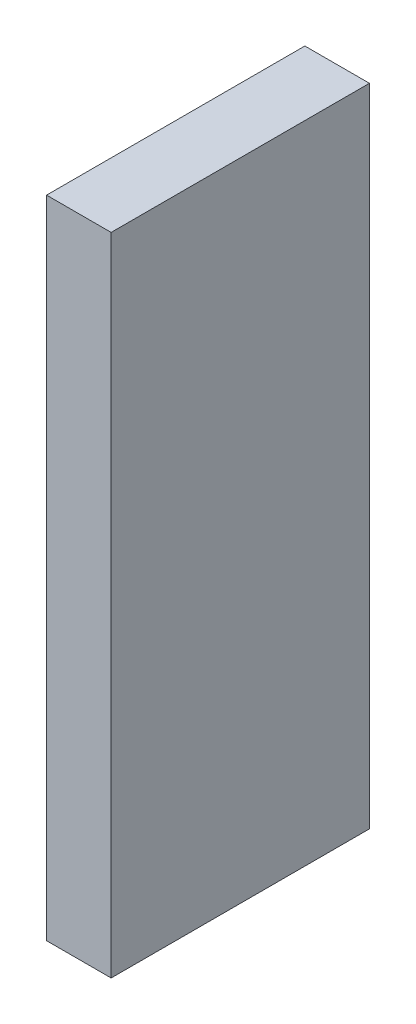
from build123d import *

# Parameters (mm, degrees)
SKETCH1_W           = 25
SKETCH1_H           = 250
BOSS_EXTRUDE1_DEPTH = 100


with BuildPart() as part:
    # Sketch1 → Boss-Extrude1 (new body)
    with BuildSketch(Plane.XY):
        with Locations((12.5, -125)):
            Rectangle(SKETCH1_W, SKETCH1_H)
    extrude(amount=BOSS_EXTRUDE1_DEPTH)


solid = part.part
